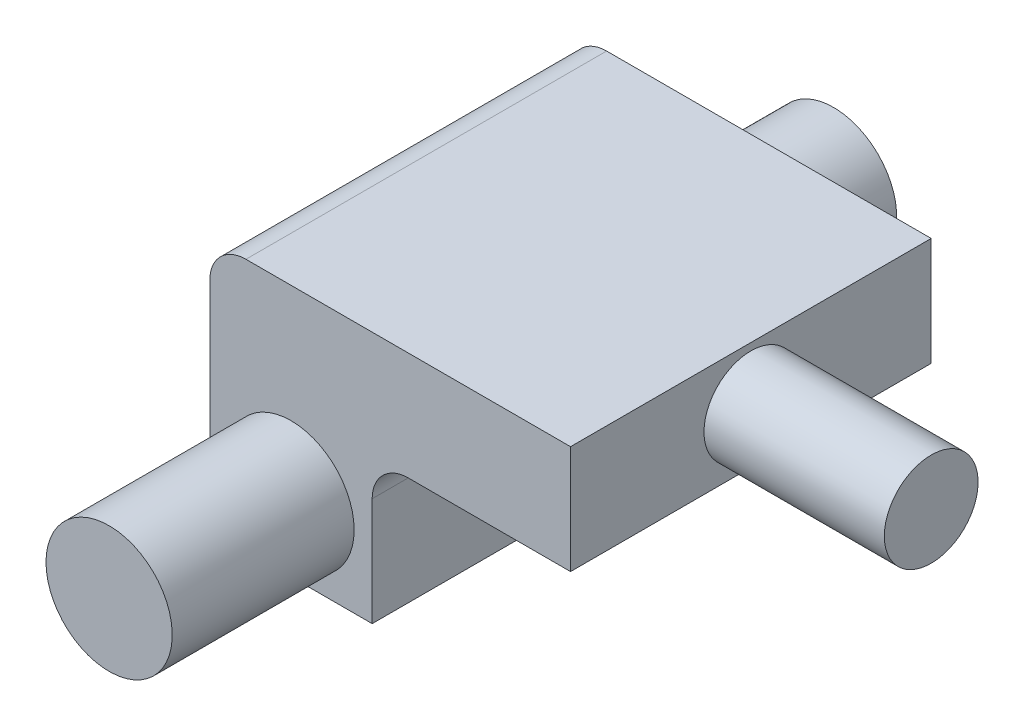
SolidWorks part; units mm, degrees
ref_plane "Front Plane" through (0, 0, 0) normal (0, 0, 1) x (1, 0, 0)
ref_plane "Top Plane" through (0, 0, 0) normal (0, 1, 0) x (1, 0, 0)
ref_plane "Right Plane" through (0, 0, 0) normal (1, 0, 0) x (0, 0, -1)
ref_plane "Plane1" through (0, -20, 0) normal (0, -1, 0) x (1, 0, 0)
sketch "Sketch1" plane through (0, -20, 0) normal (0, -1, 0) x (1, 0, 0)
  line L0 (-22.5, -50) -> (77.5, -50)
  line L1 (77.5, -50) -> (77.5, 50)
  line L2 (77.5, 50) -> (-22.5, 50)
  line L3 (-22.5, 50) -> (-22.5, -50)
extrude "Boss-Extrude1" add sketch "Sketch1" against normal blind 70
sketch "Sketch2" plane through (0, 0, -50) normal (0, 0, -1) x (-1, 0, 0)
  line L0 (-77.5, -20) -> (-22.5, -20)
  line L1 (-22.5, -20) -> (-22.5, 20)
  line L2 (-22.5, 20) -> (-77.5, 20)
  line L3 (-77.5, 20) -> (-77.5, -20)
extrude "Cut-Extrude1" cut sketch "Sketch2" against normal through all
ref_plane "Plane2" through (0, 0, 0) normal (0, 0, -1) x (-1, 0, 0)
sketch "Sketch3" plane through (0, 0, 0) normal (0, 0, -1) x (-1, 0, 0)
  line L0 (-127.5, 48) -> (-127.5, 35)
  line L1 (-127.5, 35) -> (-77.5, 35)
  line L2 (-77.5, 35) -> (-77.5, 48)
  line L3 (-77.5, 48) -> (-127.5, 48)
  line L4 (-127.5, 35) -> (-77.5, 35) construction
revolve "Revolve1" add sketch "Sketch3" angle 360 about L4
ref_plane "Plane3" through (0, 0, 0) normal (0, -1, 0) x (1, 0, 0)
sketch "Sketch4" plane through (0, 0, 0) normal (0, -1, 0) x (1, 0, 0)
  line L0 (17.5, -50) -> (0, -50)
  line L1 (0, -50) -> (0, -100.435)
  line L2 (0, -100.435) -> (17.5, -100.435)
  line L3 (17.5, -100.435) -> (17.5, -50)
  line L4 (0, -50) -> (0, -100.435) construction
revolve "Revolve2" add sketch "Sketch4" angle 360 about L4
sketch "Sketch5" plane through (0, 0, 0) normal (0, -1, 0) x (1, 0, 0)
  line L0 (17.5, 100.435) -> (0, 100.435)
  line L1 (0, 100.435) -> (0, 50)
  line L2 (0, 50) -> (17.5, 50)
  line L3 (17.5, 50) -> (17.5, 100.435)
  line L4 (0, 100.435) -> (0, 50) construction
revolve "Revolve3" add sketch "Sketch5" angle 360 about L4
fillet "Fillet1" radius 10 2 edges at (-22.5, 50, 0) (22.5, 20, 0)
